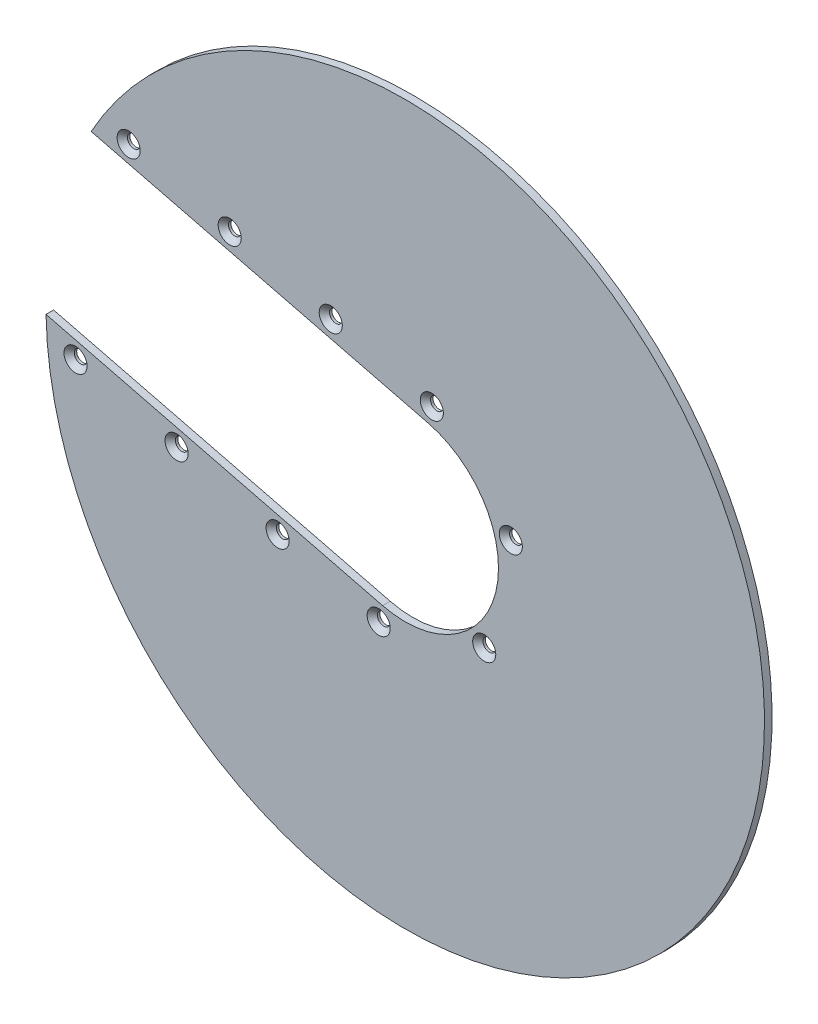
SolidWorks part; units mm, degrees
material "不锈钢板8/304"
ref_plane "Front Plane" through (0, 0, 0) normal (0, 0, 1) x (1, 0, 0)
ref_plane "Top Plane" through (0, 0, 0) normal (0, 1, 0) x (1, 0, 0)
ref_plane "Right Plane" through (0, 0, 0) normal (1, 0, 0) x (0, 0, -1)
sketch "Sketch1" plane through (0, 0, 0) normal (0, 0, 1) x (1, 0, 0)
  line L0 (-141.2544, 0) -> (0, 0) construction
  line L1 (0, 0) -> (-167.2595, 41.7025) construction
  line L2 (23.8293, 95.5741) -> (-331.7785, 184.2371)
  line L3 (-23.8293, -95.5741) -> (-379.4371, -6.9112)
  arc A0 (-379.4371, -6.9112) -> (-331.7785, 184.2371) centre (0, 0) ccw
  arc A2 (-23.8293, -95.5741) -> (23.8293, 95.5741) centre (0, 0) ccw
  dimension "D1" = 759
  dimension "D2" = 197
  dimension "D3" = 14
extrude "Boss-Extrude1" add sketch "Sketch1" along normal blind 8
sketch "Sketch2" plane through (0, 0, 8) normal (0, 0, 1) x (1, 0, 0)
  line L0 (0, 0) -> (39.6607, 159.0705) construction
  line L1 (-331.7785, 184.2371) -> (23.8293, 95.5741) construction
  circle A0 centre (0, 0) radius 116 construction
  circle A1 centre (28.0629, 112.5543) radius 12.5
  dimension "D1" = 232
  dimension "D2" = 25
sketch "Sketch3" plane through (0, 0, 0) normal (0, 0, -1) x (-1, 0, 0)
  circle A0 centre (-28.0629, 112.5543) radius 6
  dimension "D1" = 12
ref_plane "Plane1" through (0, 0, 0) normal (-0.2419, -0.9703, 0) x (-0.9703, 0.2419, 0)
sketch "Sketch4" plane through (0, 0, 8) normal (0, 0, 1) x (1, 0, 0)
  line L0 (0, 0) -> (34.8824, 139.9056) construction
  line L1 (0, 0) -> (138.603, 39.7438) construction
  line L2 (0, 0) -> (103.7206, -100.1618) construction
  line L3 (0, 0) -> (-34.8824, -139.9056) construction
  line L4 (28.0629, 112.5543) -> (-78.6696, 139.1657) construction
  line L5 (-78.6696, 139.1657) -> (-185.4021, 165.7771) construction
  line L6 (-185.4021, 165.7771) -> (-292.1346, 192.3885) construction
  line L7 (0, 0) -> (-292.1346, 72.8373) construction
  line L8 (-28.0629, -112.5543) -> (-134.7955, -85.9429) construction
  line L9 (-134.7955, -85.9429) -> (-241.528, -59.3315) construction
  line L10 (-241.528, -59.3315) -> (-348.2605, -32.7201) construction
  circle A0 centre (0, 0) radius 116 construction
  point P11 (0, 0)
  dimension "D1" = 232
  dimension "D2" = 4
  dimension "D3" = 110
  dimension "D4" = 110
  dimension "D5" = 110
hole_wizard "Hole size (per %) for Type 1 hex socket Torx semi-countersunk screw" positions "Sketch5" profile "Sketch6" countersink size "M12" standard "GB" end condition through all
sketch "Sketch5" plane through (0, 0, 8) normal (0, 0, 1) x (1, 0, 0)
  line L0 (0, 0) -> (138.603, 39.7438) construction
  line L1 (0, 0) -> (103.7206, -100.1618) construction
  circle A0 centre (0, 0) radius 116 construction
  point P0 (-292.1346, 192.3885)
  point P3 (-185.4021, 165.7771)
  point P6 (-78.6696, 139.1657)
  point P9 (28.0629, 112.5543)
  point P12 (111.5064, 31.9739)
  point P18 (83.4434, -80.5804)
  point P22 (-28.0629, -112.5543)
  point P25 (-134.7955, -85.9429)
  point P28 (-241.528, -59.3315)
  point P31 (-348.2605, -32.7201)
sketch "Sketch6" plane through (-292.1346, 192.3885, 8) normal (1, 0, 0) x (0, -1, 0)
  line L0 (0, 0) -> (0, 8)
  line L1 (0, 8) -> (6.75, 8)
  line L2 (6.75, 8) -> (6.75, 5.45)
  line L3 (6.75, 5.45) -> (12.2, 0)
  line L5 (12.2, 0) -> (0, 0)
  line L6 (-6.75, 5.45) -> (-12.2, 0) construction
  line L11 (0, -6.35) -> (0, 107.95) construction
  dimension "通孔孔直径" = 13.5
  dimension "通孔孔深度" = 8
  dimension "近端锥形沉头孔直径" = 24.4
  dimension "近端锥形沉头孔角度" = 90
